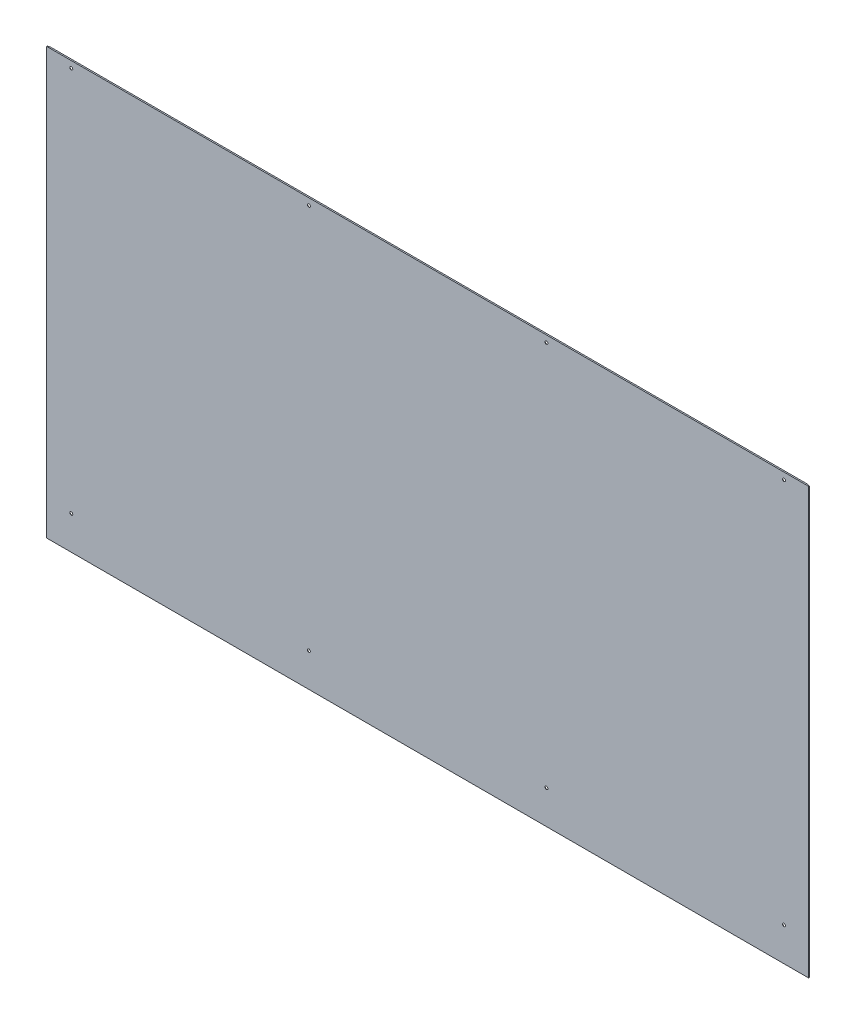
from build123d import *

# Parameters (mm, degrees)
SKETCH_1_W                    = 1700
SKETCH_1_H                    = 950
EXTRUDE_1_DEPTH               = 3
SKETCH_2_R                    = 3.25
CUT_EXTRUDE_1_DEPTH           = 3
CUT_EXTRUDE_1_DRAFT           = 45
CUT_EXTRUDE_1_PROFILE_2_DEPTH = 3
CUT_EXTRUDE_1_PROFILE_2_DRAFT = 45
CUT_EXTRUDE_1_PROFILE_3_DEPTH = 3
CUT_EXTRUDE_1_PROFILE_3_DRAFT = 45
CUT_EXTRUDE_1_PROFILE_4_DEPTH = 3
CUT_EXTRUDE_1_PROFILE_4_DRAFT = 45
CUT_EXTRUDE_1_PROFILE_5_DEPTH = 3
CUT_EXTRUDE_1_PROFILE_5_DRAFT = 45
CUT_EXTRUDE_1_PROFILE_6_DEPTH = 3
CUT_EXTRUDE_1_PROFILE_6_DRAFT = 45
CUT_EXTRUDE_1_PROFILE_7_DEPTH = 3
CUT_EXTRUDE_1_PROFILE_7_DRAFT = 45
CUT_EXTRUDE_1_PROFILE_8_DEPTH = 3
CUT_EXTRUDE_1_PROFILE_8_DRAFT = 45
CUT_EXTRUDE_2_DEPTH           = 1275.758408484


with BuildPart() as part:
    # 草图1 → 凸台-拉伸1 (new body)
    with BuildSketch(Plane.XY):
        Rectangle(SKETCH_1_W, SKETCH_1_H)
    extrude(amount=EXTRUDE_1_DEPTH)


with BuildPart() as cut_extrude_1_tool:
    # 草图2 → 切除-拉伸1 (with draft: the straight prism first)
    with BuildSketch(Plane.XY.offset(3)):
        with Locations((-795, 460)):
            Circle(SKETCH_2_R)
    extrude(amount=-CUT_EXTRUDE_1_DEPTH)
    # 切除-拉伸1: the draft: its side faces are tilted about the plane it starts from
    cut_extrude_1_sides = [cut_extrude_1_tool.faces().sort_by_distance(p)[0] for p in [
        (-798.25, 460, 1.5),
    ]]
    draft(cut_extrude_1_sides, Plane.XY.offset(3), CUT_EXTRUDE_1_DRAFT)


with BuildPart() as part_1:
    add(part.part)

    # 切除-拉伸1: cut by cut_extrude_1_tool
    add(cut_extrude_1_tool.part, mode=Mode.SUBTRACT)


with BuildPart() as cut_extrude_1_profile_2_tool:
    # 草图2 → 切除-拉伸1 profile 2 (with draft: the straight prism first)
    with BuildSketch(Plane.XY.offset(3)):
        with Locations((-265, 460)):
            Circle(SKETCH_2_R)
    extrude(amount=-CUT_EXTRUDE_1_PROFILE_2_DEPTH)
    # 切除-拉伸1 profile 2: the draft: its side faces are tilted about the plane it starts from
    cut_extrude_1_profile_2_sides = [cut_extrude_1_profile_2_tool.faces().sort_by_distance(p)[0] for p in [
        (-268.25, 460, 1.5),
    ]]
    draft(cut_extrude_1_profile_2_sides, Plane.XY.offset(3), CUT_EXTRUDE_1_PROFILE_2_DRAFT)


with BuildPart() as part_2:
    add(part_1.part)

    # 切除-拉伸1 profile 2: cut by cut_extrude_1_profile_2_tool
    add(cut_extrude_1_profile_2_tool.part, mode=Mode.SUBTRACT)


with BuildPart() as cut_extrude_1_profile_3_tool:
    # 草图2 → 切除-拉伸1 profile 3 (with draft: the straight prism first)
    with BuildSketch(Plane.XY.offset(3)):
        with Locations((265, 460)):
            Circle(SKETCH_2_R)
    extrude(amount=-CUT_EXTRUDE_1_PROFILE_3_DEPTH)
    # 切除-拉伸1 profile 3: the draft: its side faces are tilted about the plane it starts from
    cut_extrude_1_profile_3_sides = [cut_extrude_1_profile_3_tool.faces().sort_by_distance(p)[0] for p in [
        (261.75, 460, 1.5),
    ]]
    draft(cut_extrude_1_profile_3_sides, Plane.XY.offset(3), CUT_EXTRUDE_1_PROFILE_3_DRAFT)


with BuildPart() as part_3:
    add(part_2.part)

    # 切除-拉伸1 profile 3: cut by cut_extrude_1_profile_3_tool
    add(cut_extrude_1_profile_3_tool.part, mode=Mode.SUBTRACT)


with BuildPart() as cut_extrude_1_profile_4_tool:
    # 草图2 → 切除-拉伸1 profile 4 (with draft: the straight prism first)
    with BuildSketch(Plane.XY.offset(3)):
        with Locations((795, 460)):
            Circle(SKETCH_2_R)
    extrude(amount=-CUT_EXTRUDE_1_PROFILE_4_DEPTH)
    # 切除-拉伸1 profile 4: the draft: its side faces are tilted about the plane it starts from
    cut_extrude_1_profile_4_sides = [cut_extrude_1_profile_4_tool.faces().sort_by_distance(p)[0] for p in [
        (791.75, 460, 1.5),
    ]]
    draft(cut_extrude_1_profile_4_sides, Plane.XY.offset(3), CUT_EXTRUDE_1_PROFILE_4_DRAFT)


with BuildPart() as part_4:
    add(part_3.part)

    # 切除-拉伸1 profile 4: cut by cut_extrude_1_profile_4_tool
    add(cut_extrude_1_profile_4_tool.part, mode=Mode.SUBTRACT)


with BuildPart() as cut_extrude_1_profile_5_tool:
    # 草图2 → 切除-拉伸1 profile 5 (with draft: the straight prism first)
    with BuildSketch(Plane.XY.offset(3)):
        with Locations((795, -400)):
            Circle(SKETCH_2_R)
    extrude(amount=-CUT_EXTRUDE_1_PROFILE_5_DEPTH)
    # 切除-拉伸1 profile 5: the draft: its side faces are tilted about the plane it starts from
    cut_extrude_1_profile_5_sides = [cut_extrude_1_profile_5_tool.faces().sort_by_distance(p)[0] for p in [
        (791.75, -400, 1.5),
    ]]
    draft(cut_extrude_1_profile_5_sides, Plane.XY.offset(3), CUT_EXTRUDE_1_PROFILE_5_DRAFT)


with BuildPart() as part_5:
    add(part_4.part)

    # 切除-拉伸1 profile 5: cut by cut_extrude_1_profile_5_tool
    add(cut_extrude_1_profile_5_tool.part, mode=Mode.SUBTRACT)


with BuildPart() as cut_extrude_1_profile_6_tool:
    # 草图2 → 切除-拉伸1 profile 6 (with draft: the straight prism first)
    with BuildSketch(Plane.XY.offset(3)):
        with Locations((265, -400)):
            Circle(SKETCH_2_R)
    extrude(amount=-CUT_EXTRUDE_1_PROFILE_6_DEPTH)
    # 切除-拉伸1 profile 6: the draft: its side faces are tilted about the plane it starts from
    cut_extrude_1_profile_6_sides = [cut_extrude_1_profile_6_tool.faces().sort_by_distance(p)[0] for p in [
        (261.75, -400, 1.5),
    ]]
    draft(cut_extrude_1_profile_6_sides, Plane.XY.offset(3), CUT_EXTRUDE_1_PROFILE_6_DRAFT)


with BuildPart() as part_6:
    add(part_5.part)

    # 切除-拉伸1 profile 6: cut by cut_extrude_1_profile_6_tool
    add(cut_extrude_1_profile_6_tool.part, mode=Mode.SUBTRACT)


with BuildPart() as cut_extrude_1_profile_7_tool:
    # 草图2 → 切除-拉伸1 profile 7 (with draft: the straight prism first)
    with BuildSketch(Plane.XY.offset(3)):
        with Locations((-265, -400)):
            Circle(SKETCH_2_R)
    extrude(amount=-CUT_EXTRUDE_1_PROFILE_7_DEPTH)
    # 切除-拉伸1 profile 7: the draft: its side faces are tilted about the plane it starts from
    cut_extrude_1_profile_7_sides = [cut_extrude_1_profile_7_tool.faces().sort_by_distance(p)[0] for p in [
        (-268.25, -400, 1.5),
    ]]
    draft(cut_extrude_1_profile_7_sides, Plane.XY.offset(3), CUT_EXTRUDE_1_PROFILE_7_DRAFT)


with BuildPart() as part_7:
    add(part_6.part)

    # 切除-拉伸1 profile 7: cut by cut_extrude_1_profile_7_tool
    add(cut_extrude_1_profile_7_tool.part, mode=Mode.SUBTRACT)


with BuildPart() as cut_extrude_1_profile_8_tool:
    # 草图2 → 切除-拉伸1 profile 8 (with draft: the straight prism first)
    with BuildSketch(Plane.XY.offset(3)):
        with Locations((-795, -400)):
            Circle(SKETCH_2_R)
    extrude(amount=-CUT_EXTRUDE_1_PROFILE_8_DEPTH)
    # 切除-拉伸1 profile 8: the draft: its side faces are tilted about the plane it starts from
    cut_extrude_1_profile_8_sides = [cut_extrude_1_profile_8_tool.faces().sort_by_distance(p)[0] for p in [
        (-798.25, -400, 1.5),
    ]]
    draft(cut_extrude_1_profile_8_sides, Plane.XY.offset(3), CUT_EXTRUDE_1_PROFILE_8_DRAFT)


with BuildPart() as part_8:
    add(part_7.part)

    # 切除-拉伸1 profile 8: cut by cut_extrude_1_profile_8_tool
    add(cut_extrude_1_profile_8_tool.part, mode=Mode.SUBTRACT)

    # 草图3 → 切除-拉伸2 (cut, through all)
    with BuildSketch(Plane.XZ.offset(475)):
        Polygon((844.401923789, 0), (850, 1.5), (850, 0), align=None)
        Polygon((-850, 1.5), (-850, 0), (-844.401923789, 0), align=None)
    extrude(amount=-CUT_EXTRUDE_2_DEPTH, mode=Mode.SUBTRACT)


solid = part_8.part
